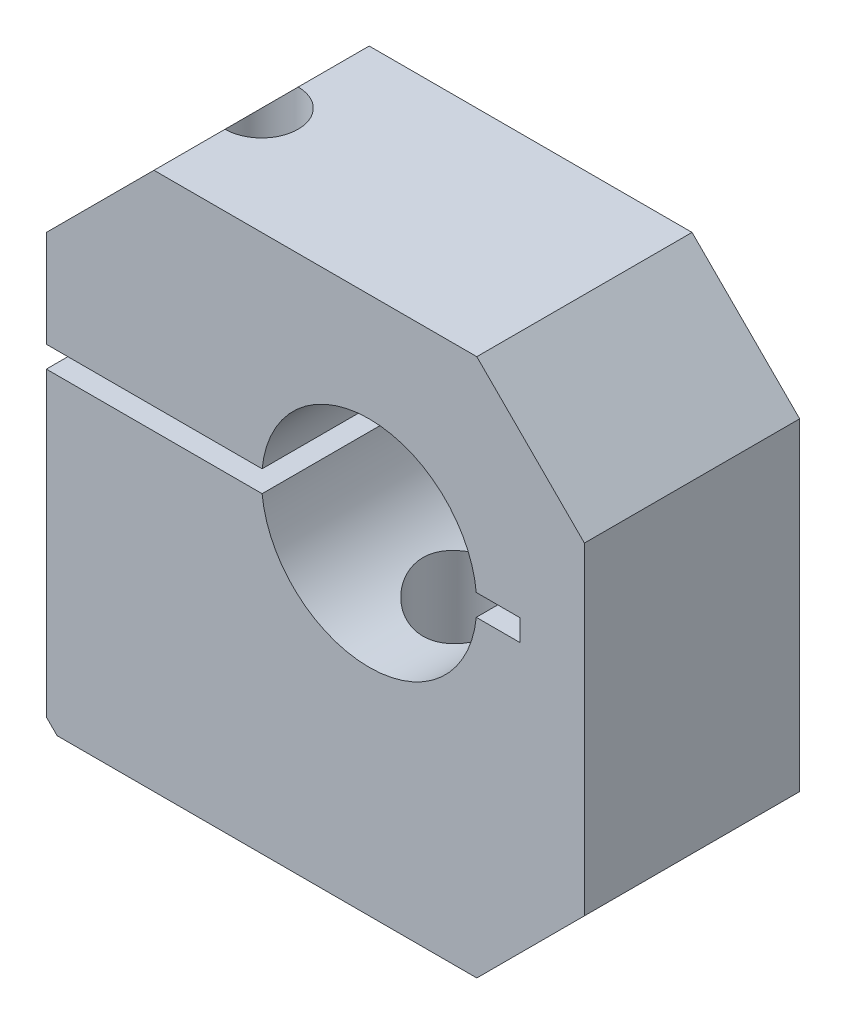
from build123d import *

# Parameters (mm, degrees)
SKETCH_1_W          = 50
SKETCH_1_H          = 50
SKETCH_1_R          = 10
EXTRUDE_1_DEPTH     = 20
CHAMFER_1_SIZE      = 10
CHAMFER_2_SIZE      = 1
HOLE_WIZARD_M8_1_D  = 6.8
SKETCH_5_R          = 4.5
CUT_EXTRUDE_1_DEPTH = 30
SKETCH_6_W          = 34.59440866
SKETCH_6_H          = 2
CUT_EXTRUDE_2_DEPTH = 44
SKETCH_7_R          = 5
CUT_EXTRUDE_5_DEPTH = 26


with BuildPart() as part:
    # 草图1 → 凸台-拉伸1 (new body)
    with BuildSketch(Plane.XY):
        Rectangle(SKETCH_1_W, SKETCH_1_H)
        with Locations((5, 5)):
            Circle(SKETCH_1_R, mode=Mode.SUBTRACT)
    extrude(amount=EXTRUDE_1_DEPTH)

    # 倒角1
    chamfer_1_edges = [part.edges().sort_by_distance(p)[0] for p in [
        (25, -25, 10),
        (-25, 25, 10),
        (25, 25, 10),
    ]]
    chamfer(chamfer_1_edges, length=CHAMFER_1_SIZE)

    # 倒角2
    chamfer_2_edges = [part.edges().sort_by_distance(p)[0] for p in [
        (-25, -25, 10),
    ]]
    chamfer(chamfer_2_edges, length=CHAMFER_2_SIZE)

    # M8 螺纹孔1 (through all)
    with Locations(Plane(origin=(0, 25, 0), x_dir=(1, 0, 0), z_dir=(0, 1, 0))):
        with Locations((-15, -10)):
            Hole(HOLE_WIZARD_M8_1_D / 2)

    # 草图5 → 切除-拉伸1 (cut)
    with BuildSketch(Plane.XZ.offset(25)):
        with Locations(Location((-15, 10, 0), (0, 0, 270))):
            Circle(SKETCH_5_R)
    extrude(amount=-CUT_EXTRUDE_1_DEPTH, mode=Mode.SUBTRACT)

    # 草图6 → 切除-拉伸2 (cut)
    with BuildSketch(Plane.ZY.offset(25)):
        with Locations((10, 5)):
            Rectangle(SKETCH_6_W, SKETCH_6_H)
    extrude(amount=-CUT_EXTRUDE_2_DEPTH, mode=Mode.SUBTRACT)

    # 草图7 → 切除-拉伸5 (cut)
    with BuildSketch(Plane.XZ.offset(25)):
        with Locations(Location((5, 10, 0), (0, 0, 270))):
            Circle(SKETCH_7_R)
    extrude(amount=-CUT_EXTRUDE_5_DEPTH, mode=Mode.SUBTRACT)


solid = part.part
